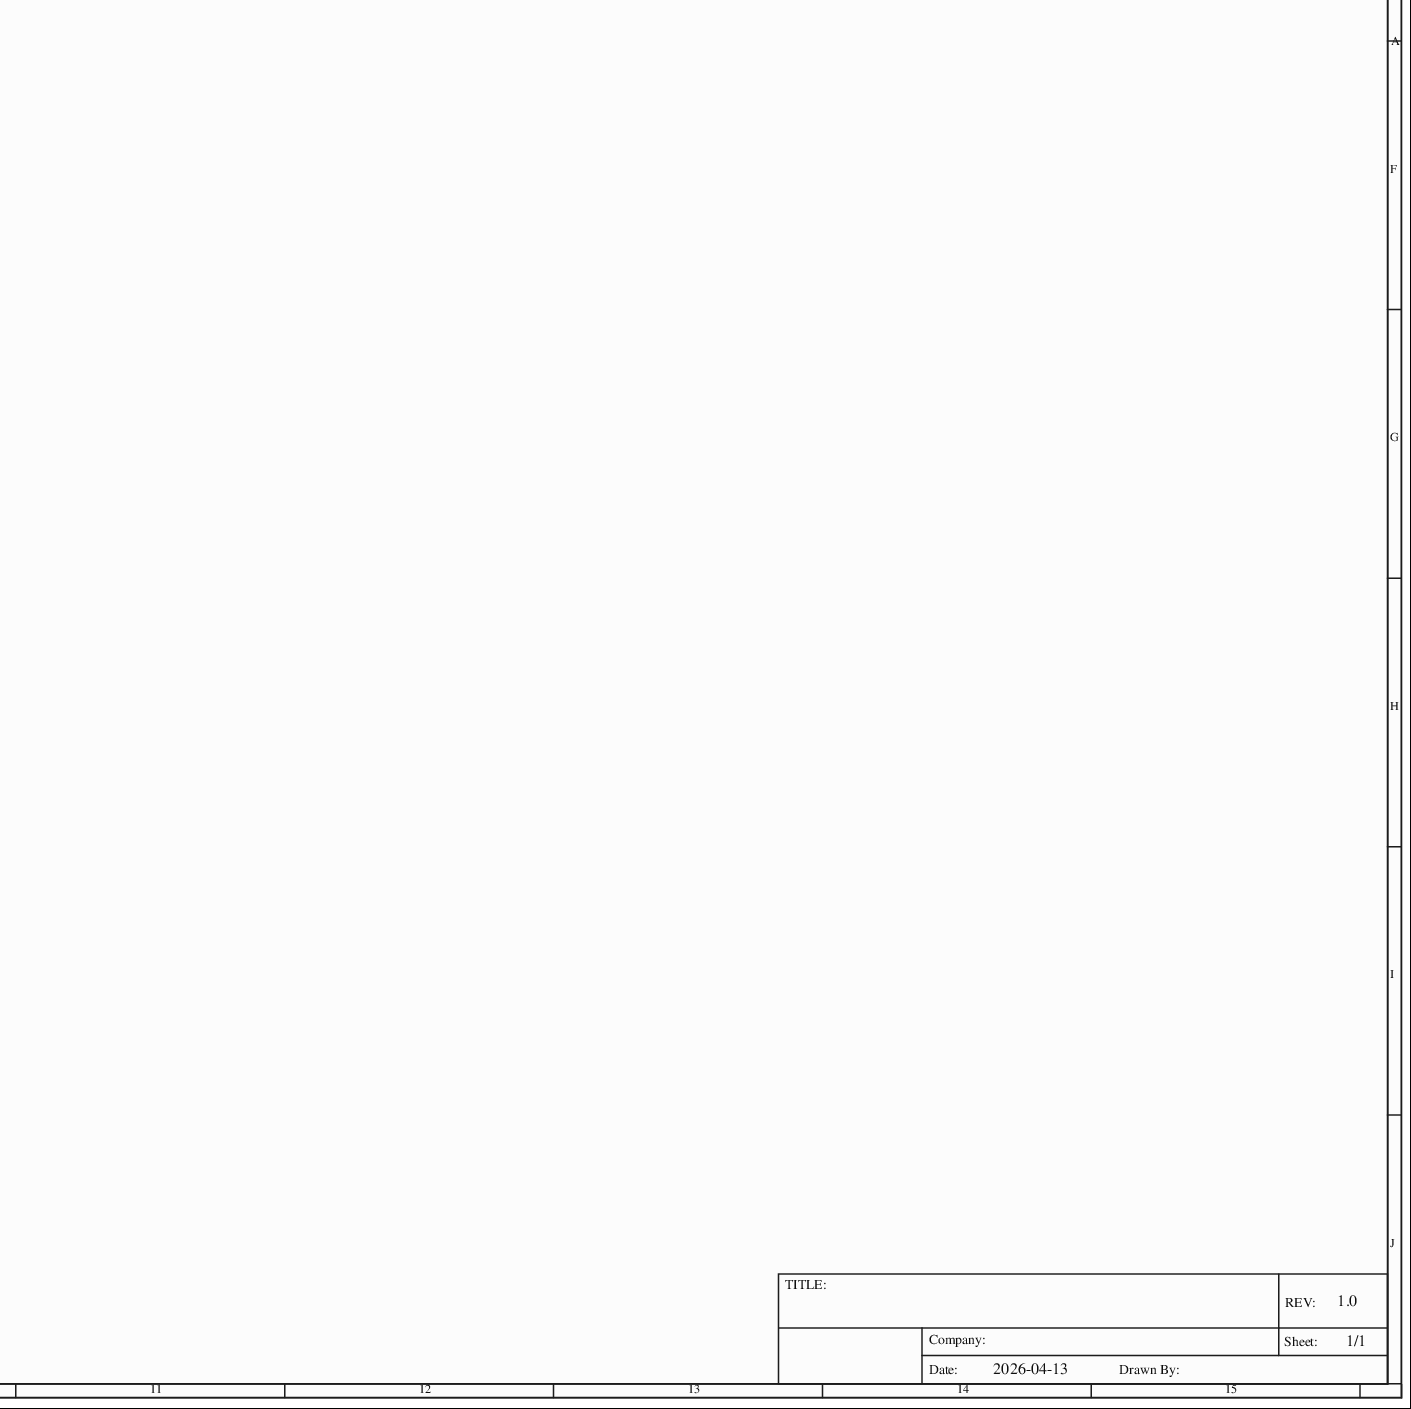
[diagram p0: MISC51540-3.schdoc, bottom right]
# Altium project MISC51540-2.PrjPcb (part 2 of 2)
## Sheet MISC51540-3.schdoc (continued)
### Blocks framed on the sheet (continued)
排针部分: PIA1 PIA2
去耦电路: C5 C17 C26 C29 C35 C37 C40 C47 C61 C62 C78 C81 C102 C107 C109 C116 C117 C122 C130 C134 C139 C5633

### Nets
1.2V: C5.2 C29.2 C37.2 C56.2 C61.2 C78.2 C102.2 C109.2 C116.2 C134.2 U1.5(VCCINT) U1.29(VCCINT) U1.37(VCCD_PLL1) U1.45(VCCINT) U1.61(VCCINT) U1.78(VCCINT) U1.102(VCCINT) U1.109(VCCD_PLL2) U1.116(VCCINT) U1.134(VCCINT) U12.2(OUT) U12.4(OUT)
2.5V: C35.2 C57.2 C107.2 U1.35(VCCA1) U1.107(VCCA2) U205.2(OUT) U205.4(OUT)
3.3V: C17.2 C25.2 C26.2 C40.2 C47.2 C59.2 C62.2 C81.2 C117.2 C122.2 C130.2 C139.2 C5633.2 JPAG.4 JZ.4(VDD) LED1.2(A) LED2.2(A) PIA1.2 PIA2.1 R1.1 R2.1 R3.1 R4.1 R5.1 RK7.2 RK8.2 RK9.2 RK10.2 RK11.2 U1.17(VCCIO1) U1.26(VCCIO2) U1.40(VCCIO3) U1.47(VCCIO3) U1.56(VCCIO4) U1.62(VCCIO4) U1.81(VCCIO5) U1.93(VCCIO6) U1.94(MSEL0) U1.97(MSEL2) U1.117(VCCIO7) U1.122(VCCIO7) U1.130(VCCIO8) U1.139(VCCIO8) U3.2(OUT) U3.4(OUT) W2516.3(IO2) W2516.7(IO3) W2516.8(VCC)
5V: C60.2 D1.1(C) PIA1.24 PIA2.23 SOUR.1 U3.3(IN) U12.3(IN) U205.3(IN)
GND: C5.1 C17.1 C25.1 C26.1 C29.1 C35.1 C37.1 C40.1 C47.1 C56.1 C57.1 C59.1 C60.1 C61.1 C62.1 C78.1 C81.1 C102.1 C107.1 C109.1 C116.1 C117.1 C122.1 C130.1 C134.1 C139.1 C5633.1 D1.2(A) JPAG.2 JPAG.10 JZ.2(GND) KEY1.1 KEY2.1 KEY3.1 KEY4.1 KEY5.1 PIA1.1 PIA1.23 PIA2.2 PIA2.24 R7.2 R921.1 RST1.1 SOUR.2 SOUR.3 U1.4(GND) U1.19(GND) U1.22(GND) U1.27(GND) U1.36(GNDA1) U1.41(GND) U1.48(GND) U1.57(GND) U1.63(GND) U1.79(GND) U1.82(GND) U1.95(GND) U1.96(MSEL1) U1.108(GNDA2) U1.118(GND) U1.123(GND) U1.131(GND) U1.140(GND) U1.145(EP) U3.1(ADJ/GND) U12.1(GND) U205.1(GND) W2516.4(GND)
ASDO: U1.6(IO,DIFFIO_L1n,(DATA1,ASDO)) W2516.5(DI/IO0)
CLK: JZ.3(OUT) U1.23(CLK1,DIFFCLK_0n)
CONF_DONE: R5.2 U1.92(CONF_DONE)
DATA0: U1.13(IO,(DATA0)) W2516.2(DO/IO1)
DCLK: U1.12(DCLK) W2516.6(CLK)
IO1: PIA2.29 U1.1(IO)
IO2: PIA2.30 U1.2(IO)
IO3: PIA2.27 U1.3(IO)
IO7: PIA2.28 U1.7(IO,VREFB1N0)
IO10: PIA2.25 U1.10(IO,DIFFIO_L4p,(DQS0L/CQ1L,DPCLK0))
IO11: PIA2.26 U1.11(IO,DIFFIO_L4n)
IO28: PIA2.21 U1.28(IO,DIFFIO_L6n)
IO30: PIA2.22 U1.30(IO,DIFFIO_L8p,(DQS1L/CQ1L#,DPCLK1))
IO31: PIA2.19 U1.31(IO,VREFB2N0)
IO32: PIA2.20 U1.32(IO,RUP1)
IO33: PIA2.17 U1.33(IO,RDN1)
IO34: PIA2.18 U1.34(IO)
IO38: PIA2.15 U1.38(IO,DIFFIO_B1p)
IO39: PIA2.16 U1.39(IO,DIFFIO_B1n)
IO42: PIA2.13 U1.42(IO,(DQS1B/CQ1B#,DPCLK2))
IO43: PIA2.14 U1.43(IO,PLL1_CLKOUTp)
IO44: PIA2.11 U1.44(IO,PLL1_CLKOUTn)
IO46: PIA2.12 U1.46(IO,VREFB3N0)
IO49: PIA2.9 U1.49(IO,DIFFIO_B9p,(DQ1B))
IO50: PIA2.10 U1.50(IO,DIFFIO_B9n,(DQ1B))
IO51: PIA2.7 U1.51(IO,DIFFIO_B10p,(DQ1B))
IO52: PIA2.8 U1.52(IO,DIFFIO_B11p)
IO53: PIA2.5 U1.53(IO,DIFFIO_B11n)
IO54: PIA2.6 U1.54(IO,DIFFIO_B12p)
IO55: PIA2.3 U1.55(IO,DIFFIO_B12n)
IO58: PIA2.4 U1.58(IO,DIFFIO_B15p,(DQ1B))
IO59: PIA1.3 U1.59(IO,DIFFIO_B16p,(DQ1B))
IO60: PIA1.4 U1.60(IO,DIFFIO_B16n,(DQ1B))
IO64: PIA1.5 U1.64(IO)
IO65: PIA1.6 U1.65(IO,VREFB4N0)
IO66: PIA1.7 U1.66(IO,RUP2,(DQ1B))
IO67: PIA1.8 U1.67(IO,RDN2,(DQ1B))
IO68: PIA1.9 U1.68(IO,DIFFIO_B20n,(DQS0B/CQ1B,DPCLK3))
IO69: PIA1.10 U1.69(IO)
IO70: PIA1.11 U1.70(IO,DIFFIO_B21p)
IO71: PIA1.12 U1.71(IO,DIFFIO_B21n)
IO72: PIA1.13 U1.72(IO,DIFFIO_B22p)
IO73: PIA1.14 U1.73(IO)
IO74: PIA1.15 U1.74(IO)
IO75: PIA1.16 U1.75(IO)
IO76: PIA1.17 U1.76(IO,RUP3)
IO77: PIA1.18 U1.77(IO,RDN3)
IO80: PIA1.19 U1.80(IO,VREFB5N0)
IO83: PIA1.20 U1.83(IO)
IO84: PIA1.21 U1.84(IO,DIFFIO_R8n)
IO85: PIA1.22 U1.85(IO,DIFFIO_R8p,(DQS1R/CQ1R#,DPCLK4))
IO86: PIA1.25 U1.86(IO,DIFFIO_R7n,(DEV_OE))
IO87: PIA1.26 U1.87(IO,DIFFIO_R7p,(DEV_CLRn))
IO98: PIA1.27 U1.98(IO,DIFFIO_R4n,(INT_DONE))
IO99: PIA1.28 U1.99(IO,DIFFIO_R4P,(CRC_ERROR))
IO100: PIA1.29 U1.100(IO)
IO101: PIA1.30 U1.101(IO,DIFFIO_R3n(nCEO))
IO103: PIA1.31 U1.103(IO,DIFFIO_R3p,(CLKUSR))
IO104: PIA1.32 U1.104(IO,(DQS0R/CQ1R,DPCLK5))
IO105: PIA1.33 U1.105(IO,VERFB6N0)
IO106: PIA1.34 U1.106(IO,DIFFIO_R1n)
IO110: PIA1.35 U1.110(IO,DIFFIO_T20p,(DQS0T/CQ1T,DPCLK6))
IO111: PIA1.36 U1.111(IO,DIFFIO_T19p)
IO112: PIA1.37 U1.112(IO,PLL2_CLKOUTn)
IO113: PIA1.38 U1.113(IO,PLL2_CLKOUTp)
IO114: PIA1.39 U1.114(IO,RUP4,(DQ1T))
IO115: PIA1.40 U1.115(IO,RDN4,(DQ1T))
IO119: PIA1.41 U1.119(IO,VREFB7N0)
IO120: PIA1.42 U1.120(IO,DIFFIO_T16n,(DQ1T))
IO121: PIA1.43 U1.121(IO,DIFFIO_T16p)
IO124: PIA1.44 U1.124(IO,DIFFIO_T13p)
IO125: R6.2 U1.125(IO)
IO126: PIA2.43 U1.126(IO,DIFFIO_T12n)
IO127: PIA2.44 U1.127(IO,DIFFIO_T12p)
IO128: PIA2.41 U1.128(IO,DIFFIO_T11n)
IO129: PIA2.42 U1.129(IO,DIFFIO_T11p)
IO132: PIA2.39 U1.132(IO,DIFFIO_T10n,(DATA2),(DQ1T))
IO133: PIA2.40 U1.133(IO,DIFFIO_T10p,(DATA3),(DQ1T))
IO135: PIA2.37 U1.135(IO,DIFFIO_T8n,(DQ1T))
IO136: PIA2.38 U1.136(IO,VREFB8N0)
IO137: PIA2.35 U1.137(IO,(DATA5),(DQ1T))
IO138: PIA2.36 U1.138(IO,(DATA6))
IO141: PIA2.33 U1.141(IO,DIFFIO_T5p)
IO142: PIA2.34 U1.142(IO,DIFFIO_T2p,(DQS1T/CQ1T#,DPCLK7))
IO143: PIA2.31 U1.143(IO,DIFFIO_T1n,(DQ1T))
IO144: PIA2.32 U1.144(IO,DIFFIO_T1p,(DM1T))
KEY1: KEY1.2 RK7.1 U1.91(CLK4,DIFFCLK_2p)
KEY2: KEY2.2 RK8.1 U1.90(CLK5,DIFFCLK_2n)
KEY3: KEY3.2 RK9.1 U1.89(CLK6,DIFFCLK_3p)
KEY4: KEY4.2 RK10.1 U1.88(CLK7,DIFFCLK_3n)
KEY5: KEY5.2 RK11.1 U1.25(CLK3,DIFFCLK_1n)
nCE: R921.2 U1.21(nCE)
nCONFIG: R1.2 RST1.2 U1.14(nCONFIG)
nCSO: U1.8(IO,DIFFIO_L2p,(FLASH_nCE,nCSO)) W2516.1(/CS)
TCK: JPAG.1 U1.16(TCK)
TDI: JPAG.9 R3.2 U1.15(TDI)
TDO: JPAG.3 U1.20(TDO)
TMS: JPAG.5 R4.2 U1.18(TMS)
NetLED1_1: LED1.1(K) R6.1
NetLED2_1: LED2.1(K) R7.1
NetR2_2: R2.2 U1.9(nSTATUS)

Not connected (* = marked no-connect by the designer): JPAG 6 7 8; JZ 1(Tri-state); U1 24(CLK2,DIFFCLK_1p)

### Notes on the sheet
- 3.3V
- 2.5V
- 1.2V
- 1
- 2
- 3
- 4
- 5
- 6
- 7
- 8
- 9
- 10
- 11
- 12
- 13
- 14
- 15
- A
- B
- C
- D
- E
- F
- G
- H
- I
- J
- TITLE:
- Company:
- Sheet:
- REV:
- 1.0
- 1/1
- Date:
- 2026-04-13
- Drawn By:

### Library data of the parts
C5 = CGA0603X7R104K500JT: Manufacturer: HRE(芯声); Convert to PCB: yes; UniqueId: gge0ab724233a2623d0; ModelId: fca5be93b99f4b5a9a2fd372d58c31d9; Device: CGA0603X7R104K500JT; Supplier: LCSC; Supplier Part: C6119867; Manufacturer Part: CGA0603X7R104K500JT; JLCPCB Part Class: Extended Part; Add into BOM: yes; SymbolName: 100nF; FootprintName: C0603; ModelName: C0603
C17 = CGA0603X7R104K500JT: Manufacturer: HRE(芯声); Convert to PCB: yes; UniqueId: gge3e3f6c4a17e9f92c; ModelId: fca5be93b99f4b5a9a2fd372d58c31d9; Device: CGA0603X7R104K500JT; Supplier: LCSC; Supplier Part: C6119867; Manufacturer Part: CGA0603X7R104K500JT; JLCPCB Part Class: Extended Part; link: https://so.szlcsc.com/global.html?k=C6119867&ref=editor; Add into BOM: yes; SymbolName: 100nF; FootprintName: C0603; ModelName: C0603
C25 = CGA0603X7R104K500JT: Manufacturer: HRE(芯声); Convert to PCB: yes; UniqueId: gge1dcd944eacf6739f; ModelId: fca5be93b99f4b5a9a2fd372d58c31d9; Device: CGA0603X7R104K500JT; Supplier: LCSC; Supplier Part: C6119867; Manufacturer Part: CGA0603X7R104K500JT; JLCPCB Part Class: Extended Part; Add into BOM: yes; SymbolName: 100nF; FootprintName: C0603; ModelName: C0603
C26 = CGA0603X7R104K500JT: Manufacturer: HRE(芯声); Convert to PCB: yes; UniqueId: ggefbb414963a23ec0e; ModelId: fca5be93b99f4b5a9a2fd372d58c31d9; Device: CGA0603X7R104K500JT; Supplier: LCSC; Supplier Part: C6119867; Manufacturer Part: CGA0603X7R104K500JT; JLCPCB Part Class: Extended Part; link: https://so.szlcsc.com/global.html?k=C6119867&ref=editor; Add into BOM: yes; SymbolName: 100nF; FootprintName: C0603; ModelName: C0603
C29 = CGA0603X7R104K500JT: Manufacturer: HRE(芯声); Convert to PCB: yes; UniqueId: ggea33bd4190d969296; ModelId: fca5be93b99f4b5a9a2fd372d58c31d9; Device: CGA0603X7R104K500JT; Supplier: LCSC; Supplier Part: C6119867; Manufacturer Part: CGA0603X7R104K500JT; JLCPCB Part Class: Extended Part; Add into BOM: yes; SymbolName: 100nF; FootprintName: C0603; ModelName: C0603
C35 = CGA0603X7R104K500JT: Manufacturer: HRE(芯声); Convert to PCB: yes; UniqueId: gge4c3bca641a64584e; ModelId: fca5be93b99f4b5a9a2fd372d58c31d9; Device: CGA0603X7R104K500JT; Supplier: LCSC; Supplier Part: C6119867; Manufacturer Part: CGA0603X7R104K500JT; JLCPCB Part Class: Extended Part; Add into BOM: yes; SymbolName: 100nF; FootprintName: C0603; ModelName: C0603
C37 = CGA0603X7R104K500JT: Manufacturer: HRE(芯声); Convert to PCB: yes; UniqueId: gge7fa45b86e39cbac6; ModelId: fca5be93b99f4b5a9a2fd372d58c31d9; Device: CGA0603X7R104K500JT; Supplier: LCSC; Supplier Part: C6119867; Manufacturer Part: CGA0603X7R104K500JT; JLCPCB Part Class: Extended Part; Add into BOM: yes; SymbolName: 100nF; FootprintName: C0603; ModelName: C0603
C40 = CGA0603X7R104K500JT: Manufacturer: HRE(芯声); Convert to PCB: yes; UniqueId: ggeef4efbbf3a1addba; ModelId: fca5be93b99f4b5a9a2fd372d58c31d9; Device: CGA0603X7R104K500JT; Supplier: LCSC; Supplier Part: C6119867; Manufacturer Part: CGA0603X7R104K500JT; JLCPCB Part Class: Extended Part; link: https://so.szlcsc.com/global.html?k=C6119867&ref=editor; Add into BOM: yes; SymbolName: 100nF; FootprintName: C0603; ModelName: C0603
C47 = CGA0603X7R104K500JT: Manufacturer: HRE(芯声); Convert to PCB: yes; UniqueId: gge8784bd8446bd5347; ModelId: fca5be93b99f4b5a9a2fd372d58c31d9; Device: CGA0603X7R104K500JT; Supplier: LCSC; Supplier Part: C6119867; Manufacturer Part: CGA0603X7R104K500JT; JLCPCB Part Class: Extended Part; link: https://so.szlcsc.com/global.html?k=C6119867&ref=editor; Add into BOM: yes; SymbolName: 100nF; FootprintName: C0603; ModelName: C0603
C56 = CGA0603X5R106K100JT: Manufacturer: HRE(芯声); Convert to PCB: yes; UniqueId: ggeb1aeb7c682b9457e; ModelId: fca5be93b99f4b5a9a2fd372d58c31d9; Device: CGA0603X5R106K100JT; Supplier: LCSC; Supplier Part: C6119842; Manufacturer Part: CGA0603X5R106K100JT; JLCPCB Part Class: Extended Part; Add into BOM: yes; SymbolName: 10uF; FootprintName: C0603; ModelName: C0603
C57 = CGA0603X5R106K100JT: Manufacturer: HRE(芯声); Convert to PCB: yes; UniqueId: ggeea8e1bc6ce9516f9; ModelId: fca5be93b99f4b5a9a2fd372d58c31d9; Device: CGA0603X5R106K100JT; Supplier: LCSC; Supplier Part: C6119842; Manufacturer Part: CGA0603X5R106K100JT; JLCPCB Part Class: Extended Part; Add into BOM: yes; SymbolName: 10uF; FootprintName: C0603; ModelName: C0603
C59 = CGA0603X5R106K100JT: Manufacturer: HRE(芯声); Convert to PCB: yes; UniqueId: gge542c9f5738b40874; ModelId: fca5be93b99f4b5a9a2fd372d58c31d9; Device: CGA0603X5R106K100JT; Supplier: LCSC; Supplier Part: C6119842; Manufacturer Part: CGA0603X5R106K100JT; JLCPCB Part Class: Extended Part; Add into BOM: yes; SymbolName: 10uF; FootprintName: C0603; ModelName: C0603
C60 = CGA0603X5R106K100JT: Manufacturer: HRE(芯声); Convert to PCB: yes; UniqueId: ggec45bc4da3ceed75e; ModelId: fca5be93b99f4b5a9a2fd372d58c31d9; Device: CGA0603X5R106K100JT; Supplier: LCSC; Supplier Part: C6119842; Manufacturer Part: CGA0603X5R106K100JT; JLCPCB Part Class: Extended Part; Add into BOM: yes; SymbolName: 10uF; FootprintName: C0603; ModelName: C0603
C61 = CGA0603X7R104K500JT: Manufacturer: HRE(芯声); Convert to PCB: yes; UniqueId: gge698b9b1cb2842f4f; ModelId: fca5be93b99f4b5a9a2fd372d58c31d9; Device: CGA0603X7R104K500JT; Supplier: LCSC; Supplier Part: C6119867; Manufacturer Part: CGA0603X7R104K500JT; JLCPCB Part Class: Extended Part; Add into BOM: yes; SymbolName: 100nF; FootprintName: C0603; ModelName: C0603
C62 = CGA0603X7R104K500JT: Manufacturer: HRE(芯声); Convert to PCB: yes; UniqueId: gge2b5a30a8139660d3; ModelId: fca5be93b99f4b5a9a2fd372d58c31d9; Device: CGA0603X7R104K500JT; Supplier: LCSC; Supplier Part: C6119867; Manufacturer Part: CGA0603X7R104K500JT; JLCPCB Part Class: Extended Part; link: https://so.szlcsc.com/global.html?k=C6119867&ref=editor; Add into BOM: yes; SymbolName: 100nF; FootprintName: C0603; ModelName: C0603
C78 = CGA0603X7R104K500JT: Manufacturer: HRE(芯声); Convert to PCB: yes; UniqueId: gge1c8932c338afe5d9; ModelId: fca5be93b99f4b5a9a2fd372d58c31d9; Device: CGA0603X7R104K500JT; Supplier: LCSC; Supplier Part: C6119867; Manufacturer Part: CGA0603X7R104K500JT; JLCPCB Part Class: Extended Part; Add into BOM: yes; SymbolName: 100nF; FootprintName: C0603; ModelName: C0603
C81 = CGA0603X7R104K500JT: Manufacturer: HRE(芯声); Convert to PCB: yes; UniqueId: ggebe4fcc6ac8c27808; ModelId: fca5be93b99f4b5a9a2fd372d58c31d9; Device: CGA0603X7R104K500JT; Supplier: LCSC; Supplier Part: C6119867; Manufacturer Part: CGA0603X7R104K500JT; JLCPCB Part Class: Extended Part; link: https://so.szlcsc.com/global.html?k=C6119867&ref=editor; Add into BOM: yes; SymbolName: 100nF; FootprintName: C0603; ModelName: C0603
C102 = CGA0603X7R104K500JT: Manufacturer: HRE(芯声); Convert to PCB: yes; UniqueId: gge00da9887cda85263; ModelId: fca5be93b99f4b5a9a2fd372d58c31d9; Device: CGA0603X7R104K500JT; Supplier: LCSC; Supplier Part: C6119867; Manufacturer Part: CGA0603X7R104K500JT; JLCPCB Part Class: Extended Part; Add into BOM: yes; SymbolName: 100nF; FootprintName: C0603; ModelName: C0603
C107 = CGA0603X7R104K500JT: Manufacturer: HRE(芯声); Convert to PCB: yes; UniqueId: gge82d5f65b0fe58dba; ModelId: fca5be93b99f4b5a9a2fd372d58c31d9; Device: CGA0603X7R104K500JT; Supplier: LCSC; Supplier Part: C6119867; Manufacturer Part: CGA0603X7R104K500JT; JLCPCB Part Class: Extended Part; Add into BOM: yes; SymbolName: 100nF; FootprintName: C0603; ModelName: C0603
C109 = CGA0603X7R104K500JT: Manufacturer: HRE(芯声); Convert to PCB: yes; UniqueId: gge1731ea11c8b72662; ModelId: fca5be93b99f4b5a9a2fd372d58c31d9; Device: CGA0603X7R104K500JT; Supplier: LCSC; Supplier Part: C6119867; Manufacturer Part: CGA0603X7R104K500JT; JLCPCB Part Class: Extended Part; Add into BOM: yes; SymbolName: 100nF; FootprintName: C0603; ModelName: C0603
C116 = CGA0603X7R104K500JT: Manufacturer: HRE(芯声); Convert to PCB: yes; UniqueId: gge9f5b62235702b252; ModelId: fca5be93b99f4b5a9a2fd372d58c31d9; Device: CGA0603X7R104K500JT; Supplier: LCSC; Supplier Part: C6119867; Manufacturer Part: CGA0603X7R104K500JT; JLCPCB Part Class: Extended Part; Add into BOM: yes; SymbolName: 100nF; FootprintName: C0603; ModelName: C0603
C117 = CGA0603X7R104K500JT: Manufacturer: HRE(芯声); Convert to PCB: yes; UniqueId: gge5cce9421618e3794; ModelId: fca5be93b99f4b5a9a2fd372d58c31d9; Device: CGA0603X7R104K500JT; Supplier: LCSC; Supplier Part: C6119867; Manufacturer Part: CGA0603X7R104K500JT; JLCPCB Part Class: Extended Part; Add into BOM: yes; SymbolName: 100nF; FootprintName: C0603; ModelName: C0603
C122 = CGA0603X7R104K500JT: Manufacturer: HRE(芯声); Convert to PCB: yes; UniqueId: gge3d3e24355e051a57; ModelId: fca5be93b99f4b5a9a2fd372d58c31d9; Device: CGA0603X7R104K500JT; Supplier: LCSC; Supplier Part: C6119867; Manufacturer Part: CGA0603X7R104K500JT; JLCPCB Part Class: Extended Part; link: https://so.szlcsc.com/global.html?k=C6119867&ref=editor; Add into BOM: yes; SymbolName: 100nF; FootprintName: C0603; ModelName: C0603
C130 = CGA0603X7R104K500JT: Manufacturer: HRE(芯声); Convert to PCB: yes; UniqueId: gge29212a6e23b95e0d; ModelId: fca5be93b99f4b5a9a2fd372d58c31d9; Device: CGA0603X7R104K500JT; Supplier: LCSC; Supplier Part: C6119867; Manufacturer Part: CGA0603X7R104K500JT; JLCPCB Part Class: Extended Part; Add into BOM: yes; SymbolName: 100nF; FootprintName: C0603; ModelName: C0603
C134 = CGA0603X7R104K500JT: Manufacturer: HRE(芯声); Convert to PCB: yes; UniqueId: gge3ddb7be29c389289; ModelId: fca5be93b99f4b5a9a2fd372d58c31d9; Device: CGA0603X7R104K500JT; Supplier: LCSC; Supplier Part: C6119867; Manufacturer Part: CGA0603X7R104K500JT; JLCPCB Part Class: Extended Part; Add into BOM: yes; SymbolName: 100nF; FootprintName: C0603; ModelName: C0603
C139 = CGA0603X7R104K500JT: Manufacturer: HRE(芯声); Convert to PCB: yes; UniqueId: ggee1a7ee9afa0f1941; ModelId: fca5be93b99f4b5a9a2fd372d58c31d9; Device: CGA0603X7R104K500JT; Supplier: LCSC; Supplier Part: C6119867; Manufacturer Part: CGA0603X7R104K500JT; JLCPCB Part Class: Extended Part; Add into BOM: yes; SymbolName: 100nF; FootprintName: C0603; ModelName: C0603
C5633 = CGA0603X7R104K500JT: Manufacturer: HRE(芯声); Convert to PCB: yes; UniqueId: gge4823bfea76416029; ModelId: fca5be93b99f4b5a9a2fd372d58c31d9; Device: CGA0603X7R104K500JT; Supplier: LCSC; Supplier Part: C6119867; Manufacturer Part: CGA0603X7R104K500JT; JLCPCB Part Class: Extended Part; link: https://so.szlcsc.com/global.html?k=C6119867&ref=editor; Add into BOM: yes; SymbolName: 100nF; FootprintName: C0603; ModelName: C0603
D1 = SMAJ5.0A: Manufacturer: Littelfuse(美国力特); Convert to PCB: yes; UniqueId: ggebe0b25424dfff157; ModelId: 7ed2c9d0a4a74bbdbba07ab4052caf5b; Device: SMAJ5.0A; Supplier: LCSC; Manufacturer Part: SMAJ5.0A; Supplier Part: C83329; JLCPCB Part Class: Extended Part; Add into BOM: yes; SymbolName: SMAJ5.0A-C83329; FootprintName: SMA_L4.3-W2.6-LS5.2-RD; ModelName: SMA_L4.3-W2.6-LS5.2-RD
JPAG = MTB10-10S: Manufacturer: MINTRON(明硕); Convert to PCB: yes; UniqueId: gge31a9ef06757d570f; Device: MTB10-10S; Supplier: LCSC; Supplier Part: C358743; Manufacturer Part: MTB10-10S; JLCPCB Part Class: Extended Part; Add into BOM: yes; SymbolName: MTB110-10S; FootprintName: IDC-TH_MTB110-10S
JZ = OT1EL89CJI-111YLC-50M: Manufacturer: YXC(扬兴晶振); Convert to PCB: yes; UniqueId: gge580d0efcced3635b; ModelId: 3a2688c8917e419f908ee8ddbc603a15; Device: OT1EL89CJI-111YLC-50M; Supplier: LCSC; Supplier Part: C7429728; Manufacturer Part: OT1EL89CJI-111YLC-50M; JLCPCB Part Class: Extended Part; Add into BOM: yes; SymbolName: 50MHz; FootprintName: OSC-SMD_4P-L5.0-W3.2-BL_7CZ-XXXXX; ModelName: OSC-SMD_4P-L5.0-W3.2-BL_7CZ-XXXXX
KEY1 = K2-1107ST-A4SW-06: 制造商: 韩国韩荣; Convert to PCB: yes; UniqueId: gge720e1b283bfbdb00; ModelId: 0116d9fe13534fa3ad56976dc35a6258; Device: K2-1107ST-A4SW-06; Supplier Part: C118141; Supplier: LCSC; Manufacturer Part: K2-1107ST-A4SW-06; Add into BOM: yes; SymbolName: K2-3.6×6.1_SMD; FootprintName: KEY-SMD_2P-L6.2-W3.6-LS8.0; ModelName: KEY-SMD_2P-L6.2-W3.6-LS8.0
KEY2 = K2-1107ST-A4SW-06: 制造商: 韩国韩荣; Convert to PCB: yes; UniqueId: ggece9f37484477e190; ModelId: 0116d9fe13534fa3ad56976dc35a6258; Device: K2-1107ST-A4SW-06; Supplier Part: C118141; Supplier: LCSC; Manufacturer Part: K2-1107ST-A4SW-06; Add into BOM: yes; SymbolName: K2-3.6×6.1_SMD; FootprintName: KEY-SMD_2P-L6.2-W3.6-LS8.0; ModelName: KEY-SMD_2P-L6.2-W3.6-LS8.0
KEY3 = K2-1107ST-A4SW-06: 制造商: 韩国韩荣; Convert to PCB: yes; UniqueId: gge980bab35a034d4fc; ModelId: 0116d9fe13534fa3ad56976dc35a6258; Device: K2-1107ST-A4SW-06; Supplier Part: C118141; Supplier: LCSC; Manufacturer Part: K2-1107ST-A4SW-06; Add into BOM: yes; SymbolName: K2-3.6×6.1_SMD; FootprintName: KEY-SMD_2P-L6.2-W3.6-LS8.0; ModelName: KEY-SMD_2P-L6.2-W3.6-LS8.0
KEY4 = K2-1107ST-A4SW-06: 制造商: 韩国韩荣; Convert to PCB: yes; UniqueId: gge58d96aa54349b1c8; ModelId: 0116d9fe13534fa3ad56976dc35a6258; Device: K2-1107ST-A4SW-06; Supplier Part: C118141; Supplier: LCSC; Manufacturer Part: K2-1107ST-A4SW-06; Add into BOM: yes; SymbolName: K2-3.6×6.1_SMD; FootprintName: KEY-SMD_2P-L6.2-W3.6-LS8.0; ModelName: KEY-SMD_2P-L6.2-W3.6-LS8.0
KEY5 = K2-1107ST-A4SW-06: 制造商: 韩国韩荣; Convert to PCB: yes; UniqueId: ggeff9343ae3dda900c; ModelId: 0116d9fe13534fa3ad56976dc35a6258; Device: K2-1107ST-A4SW-06; Supplier Part: C118141; Supplier: LCSC; Manufacturer Part: K2-1107ST-A4SW-06; Add into BOM: yes; SymbolName: K2-3.6×6.1_SMD; FootprintName: KEY-SMD_2P-L6.2-W3.6-LS8.0; ModelName: KEY-SMD_2P-L6.2-W3.6-LS8.0
LED1 = NCD0603Y2: Manufacturer: 国星光电; Convert to PCB: yes; UniqueId: gge5cc62ecb4d8d0cb4; ModelId: 1f0d29a91be547639d425604e9b96ebb; Device: NCD0603Y2; Supplier: LCSC; Manufacturer Part: NCD0603Y2; Supplier Part: C89811; JLCPCB Part Class: Extended Part; Add into BOM: yes; SymbolName: FC-1608YXK-585F08; FootprintName: LED0603-RD; ModelName: LED0603-RD
LED2 = NCD0603Y2: Manufacturer: 国星光电; Convert to PCB: yes; UniqueId: gge8315dec841cc40ed; ModelId: 1f0d29a91be547639d425604e9b96ebb; Device: NCD0603Y2; Supplier: LCSC; Manufacturer Part: NCD0603Y2; Supplier Part: C89811; JLCPCB Part Class: Extended Part; Add into BOM: yes; SymbolName: FC-1608YXK-585F08; FootprintName: LED0603-RD; ModelName: LED0603-RD
PIA1 = X6521WV-2x22H-C60D30: Manufacturer: XKB Connection(中国星坤); Convert to PCB: yes; UniqueId: ggef922af296db4e291; Device: X6521WV-2x22H-C60D30; Supplier: LCSC; Supplier Part: C725894; Manufacturer Part: X6521WV-2x22H-C60D30; JLCPCB Part Class: Extended Part; Add into BOM: yes; SymbolName: X6521WV-2×22H-C30D60; FootprintName: HDR-TH_44P-2.54-V-M-R2-C22-S2.54
PIA2 = X6521WV-2x22H-C60D30: Manufacturer: XKB Connection(中国星坤); Convert to PCB: yes; UniqueId: gged018c0eec35e7a5e; Device: X6521WV-2x22H-C60D30; Supplier: LCSC; Supplier Part: C725894; Manufacturer Part: X6521WV-2x22H-C60D30; JLCPCB Part Class: Extended Part; Add into BOM: yes; SymbolName: X6521WV-2×22H-C30D60; FootprintName: HDR-TH_44P-2.54-V-M-R2-C22-S2.54
R1 = RC0402FR-0710KL: Manufacturer: YAGEO(国巨); Convert to PCB: yes; UniqueId: gge8c3ff140cf07b4f4; Device: RC0402FR-0710KL; Supplier: LCSC; Manufacturer Part: RC0402FR-0710KL; Supplier Part: C60490; JLCPCB Part Class: Extended Part; link: https://so.szlcsc.com/global.html?k=C60490&ref=editor; Add into BOM: yes; SymbolName: 10kΩ; FootprintName: R0402
R2 = RC0402FR-0710KL: Manufacturer: YAGEO(国巨); Convert to PCB: yes; UniqueId: gge7c5f0b0b987907ab; Device: RC0402FR-0710KL; Supplier: LCSC; Manufacturer Part: RC0402FR-0710KL; Supplier Part: C60490; JLCPCB Part Class: Extended Part; Add into BOM: yes; SymbolName: 10kΩ; FootprintName: R0402
R3 = RC0402FR-0710KL: Manufacturer: YAGEO(国巨); Convert to PCB: yes; UniqueId: ggee1e3f75c55ba9fa7; Device: RC0402FR-0710KL; Supplier: LCSC; Manufacturer Part: RC0402FR-0710KL; Supplier Part: C60490; JLCPCB Part Class: Extended Part; link: https://so.szlcsc.com/global.html?k=C60490&ref=editor; Add into BOM: yes; SymbolName: 10kΩ; FootprintName: R0402
R4 = RC0402FR-0710KL: Manufacturer: YAGEO(国巨); Convert to PCB: yes; UniqueId: gged94606aae0617f99; Device: RC0402FR-0710KL; Supplier: LCSC; Manufacturer Part: RC0402FR-0710KL; Supplier Part: C60490; JLCPCB Part Class: Extended Part; link: https://so.szlcsc.com/global.html?k=C60490&ref=editor; Add into BOM: yes; SymbolName: 10kΩ; FootprintName: R0402
R5 = RC0402FR-0710KL: Manufacturer: YAGEO(国巨); Convert to PCB: yes; UniqueId: gge6b8e686a2eae244f; Device: RC0402FR-0710KL; Supplier: LCSC; Manufacturer Part: RC0402FR-0710KL; Supplier Part: C60490; JLCPCB Part Class: Extended Part; link: https://so.szlcsc.com/global.html?k=C60490&ref=editor; Add into BOM: yes; SymbolName: 10kΩ; FootprintName: R0402
R6 = ARG05BTC5000: Manufacturer: Viking(光颉); Convert to PCB: yes; UniqueId: ggea8e5b6c1febceacb; ModelId: 1f8f9bfd8e2b427398b06535d781678a; Device: ARG05BTC5000; Supplier: LCSC; Supplier Part: C2828711; Manufacturer Part: ARG05BTC5000; JLCPCB Part Class: Extended Part; Add into BOM: yes; SymbolName: 500Ω; FootprintName: R0805; ModelName: R0805
R7 = ARG05BTC5000: Manufacturer: Viking(光颉); Convert to PCB: yes; UniqueId: gged5f28d2cfea9fa4c; ModelId: 1f8f9bfd8e2b427398b06535d781678a; Device: ARG05BTC5000; Supplier: LCSC; Supplier Part: C2828711; Manufacturer Part: ARG05BTC5000; JLCPCB Part Class: Extended Part; Add into BOM: yes; SymbolName: 500Ω; FootprintName: R0805; ModelName: R0805
R921 = RC0402FR-0710KL: Manufacturer: YAGEO(国巨); Convert to PCB: yes; UniqueId: gge2de88fa165fe6e76; Device: RC0402FR-0710KL; Supplier: LCSC; Manufacturer Part: RC0402FR-0710KL; Supplier Part: C60490; JLCPCB Part Class: Extended Part; link: https://so.szlcsc.com/global.html?k=C60490&ref=editor; Add into BOM: yes; SymbolName: 10kΩ; FootprintName: R0402
RK7 = RC0402FR-0710KL: Manufacturer: YAGEO(国巨); Convert to PCB: yes; UniqueId: ggea8f7886943958ce8; Device: RC0402FR-0710KL; Supplier: LCSC; Manufacturer Part: RC0402FR-0710KL; Supplier Part: C60490; JLCPCB Part Class: Extended Part; Add into BOM: yes; SymbolName: 10kΩ; FootprintName: R0402
RK8 = RC0402FR-0710KL: Manufacturer: YAGEO(国巨); Convert to PCB: yes; UniqueId: ggeb9e6bfeb1d8ee47b; Device: RC0402FR-0710KL; Supplier: LCSC; Manufacturer Part: RC0402FR-0710KL; Supplier Part: C60490; JLCPCB Part Class: Extended Part; Add into BOM: yes; SymbolName: 10kΩ; FootprintName: R0402
RK9 = RC0402FR-0710KL: Manufacturer: YAGEO(国巨); Convert to PCB: yes; UniqueId: ggedeb83df13b810bd3; Device: RC0402FR-0710KL; Supplier: LCSC; Manufacturer Part: RC0402FR-0710KL; Supplier Part: C60490; JLCPCB Part Class: Extended Part; Add into BOM: yes; SymbolName: 10kΩ; FootprintName: R0402
RK10 = RC0402FR-0710KL: Manufacturer: YAGEO(国巨); Convert to PCB: yes; UniqueId: gge030db1d844a29ee1; Device: RC0402FR-0710KL; Supplier: LCSC; Manufacturer Part: RC0402FR-0710KL; Supplier Part: C60490; JLCPCB Part Class: Extended Part; Add into BOM: yes; SymbolName: 10kΩ; FootprintName: R0402
RK11 = RC0402FR-0710KL: Manufacturer: YAGEO(国巨); Convert to PCB: yes; UniqueId: ggec7da0be3da2bb216; Device: RC0402FR-0710KL; Supplier: LCSC; Manufacturer Part: RC0402FR-0710KL; Supplier Part: C60490; JLCPCB Part Class: Extended Part; Add into BOM: yes; SymbolName: 10kΩ; FootprintName: R0402
RST1 = K2-1107ST-A4SW-06: 制造商: 韩国韩荣; Convert to PCB: yes; UniqueId: ggec1e5a143af4c2ccd; ModelId: 0116d9fe13534fa3ad56976dc35a6258; Device: K2-1107ST-A4SW-06; Supplier Part: C118141; Supplier: LCSC; Manufacturer Part: K2-1107ST-A4SW-06; Add into BOM: yes; SymbolName: K2-3.6×6.1_SMD; FootprintName: KEY-SMD_2P-L6.2-W3.6-LS8.0; ModelName: KEY-SMD_2P-L6.2-W3.6-LS8.0
SOUR = DC-005-2.0: Manufacturer: HanElectricity(瀚源); Convert to PCB: yes; UniqueId: gge73902981697d1038; ModelId: 1536c764fdf948548c94e43221d5c3cd; Device: DC-005-2.0; Supplier: LCSC; Supplier Part: C22459640; Manufacturer Part: DC-005-2.0; JLCPCB Part Class: Extended Part; Add into BOM: yes; SymbolName: DC-005-2.0_C22459640; FootprintName: DC-IN-TH_DC-005-2.0_C22459640; ModelName: DC-IN-TH_DC-005-2.0_C22459640
U1 = EP4CE6E22C8N: Manufacturer: Intel/Altera; Convert to PCB: yes; UniqueId: gge5b6e8609bed79fcf; Device: EP4CE6E22C8N; Supplier Part: C36238; Supplier: LCSC; Manufacturer Part: EP4CE6E22C8N; JLCPCB Part Class: Extended Part; link: https://so.szlcsc.com/global.html?k=C36238&ref=editor; Add into BOM: yes; SymbolName: EP4CE6E22C8N; FootprintName: PQFP-144_L20.0-W20.0-P0.50-LS22.0-BL-EP
U3 = TLV1117LV33DCYR: Manufacturer: TI(德州仪器); Convert to PCB: yes; UniqueId: gge23fb0b0865d9e337; Device: TLV1117LV33DCYR; Supplier: LCSC; Manufacturer Part: TLV1117LV33DCYR; Supplier Part: C15578; JLCPCB Part Class: Extended Part; Add into BOM: yes; SymbolName: TLV1117LV33DCYR; FootprintName: SOT-223_L6.7-W3.5-P2.30-BR
U12 = TLV1117LV12DCYR: Manufacturer: TI(德州仪器); Convert to PCB: yes; UniqueId: ggece97e5d682c0c8b4; Device: TLV1117LV12DCYR; Supplier: LCSC; Manufacturer Part: TLV1117LV12DCYR; Supplier Part: C80106; JLCPCB Part Class: Extended Part; Add into BOM: yes; SymbolName: TLV1117LV12DCYR; FootprintName: SOT-223-4_L6.5-W3.5-P2.30-LS7.0-BR
U205 = TLV1117LV25DCYR: Manufacturer: TI(德州仪器); Convert to PCB: yes; UniqueId: gge4380164c9cbb7453; Device: TLV1117LV25DCYR; Supplier: LCSC; Supplier Part: C507263; Manufacturer Part: TLV1117LV25DCYR; JLCPCB Part Class: Extended Part; Add into BOM: yes; SymbolName: TLV1117LV25DCYR; FootprintName: SOT-223-3_L6.5-W3.4-P2.30-LS7.0-BR
W2516 = W25Q16JVSSIQ: Manufacturer: Winbond(华邦); Convert to PCB: yes; UniqueId: ggeec20e417d5d789f6; Device: W25Q16JVSSIQ; Supplier: LCSC; Manufacturer Part: W25Q16JVSSIQ; Supplier Part: C82317; JLCPCB Part Class: Extended Part; Add into BOM: yes; SymbolName: W25Q16JVSSIQ; FootprintName: SOIC-8_L5.3-W5.3-P1.27-LS8.0-BL